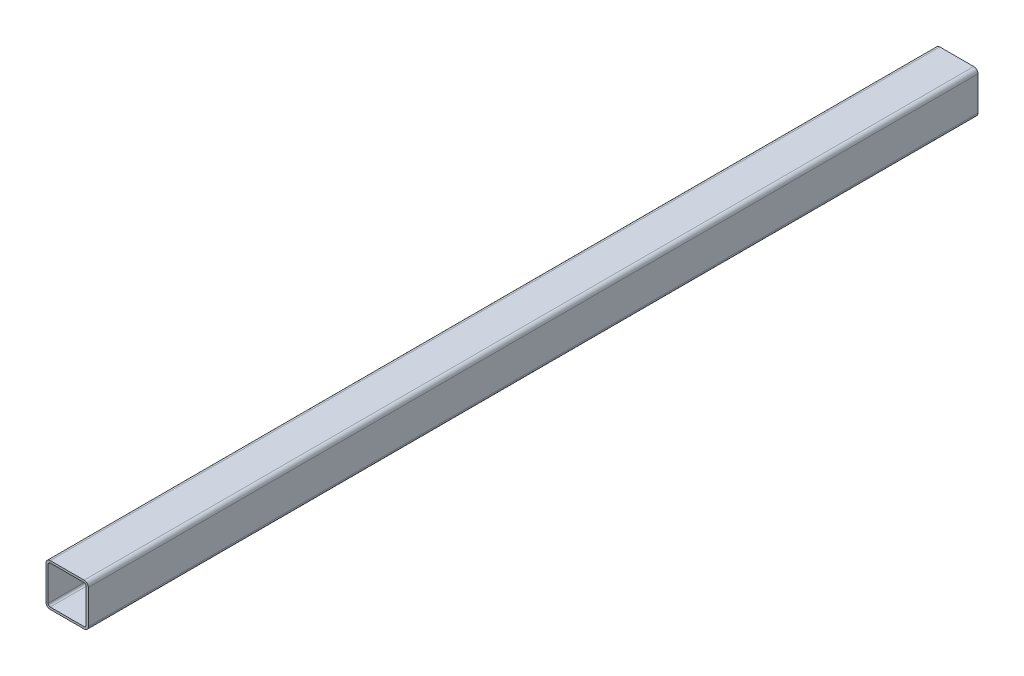
SolidWorks part; units mm, degrees
ref_plane "Front Plane" through (0, 0, 0) normal (0, 0, 1) x (1, 0, 0)
ref_plane "Top Plane" through (0, 0, 0) normal (0, 1, 0) x (1, 0, 0)
ref_plane "Right Plane" through (0, 0, 0) normal (1, 0, 0) x (0, 0, -1)
sketch "Sketch 1" plane through (0, 0, 0) normal (0, 0, 1) x (1, 0, 0)
  line L0 (0, 96.8978) -> (0, -107.4818) construction
  line L1 (-129.1971, 0) -> (137.9562, 0) construction
  line L2 (0, 50) -> (-40, 50)
  line L3 (-50, 40) -> (-50, 0)
  line L4 (0, 45) -> (-40, 45)
  line L5 (-45, 40) -> (-45, 0)
  line L6 (-45, -40) -> (-45, 0)
  line L7 (40, -45) -> (-40, -45)
  line L8 (-50, -40) -> (-50, 0)
  line L9 (40, -50) -> (-40, -50)
  line L10 (50, -40) -> (50, 0)
  line L11 (45, -40) -> (45, 0)
  line L12 (45, 40) -> (45, 0)
  line L13 (0, 45) -> (40, 45)
  line L14 (50, 40) -> (50, 0)
  line L15 (0, 50) -> (40, 50)
  arc A0 (-40, 50) -> (-50, 40) centre (-40, 40) ccw
  arc A1 (-40, 45) -> (-45, 40) centre (-40, 40) ccw
  arc A2 (-40, -45) -> (-45, -40) centre (-40, -40) cw
  arc A3 (-40, -50) -> (-50, -40) centre (-40, -40) cw
  arc A4 (40, -50) -> (50, -40) centre (40, -40) ccw
  arc A5 (40, -45) -> (45, -40) centre (40, -40) ccw
  arc A6 (40, 45) -> (45, 40) centre (40, 40) cw
  arc A7 (40, 50) -> (50, 40) centre (40, 40) cw
  point P34 (0, -50)
  point P35 (0, -45)
  dimension "D3" = 10
  dimension "D1" = 100
  dimension "D2" = 100
  dimension "D4" = 5
extrude "Boss-Extrude 1" add sketch "Sketch 1" along normal mid plane 2100
